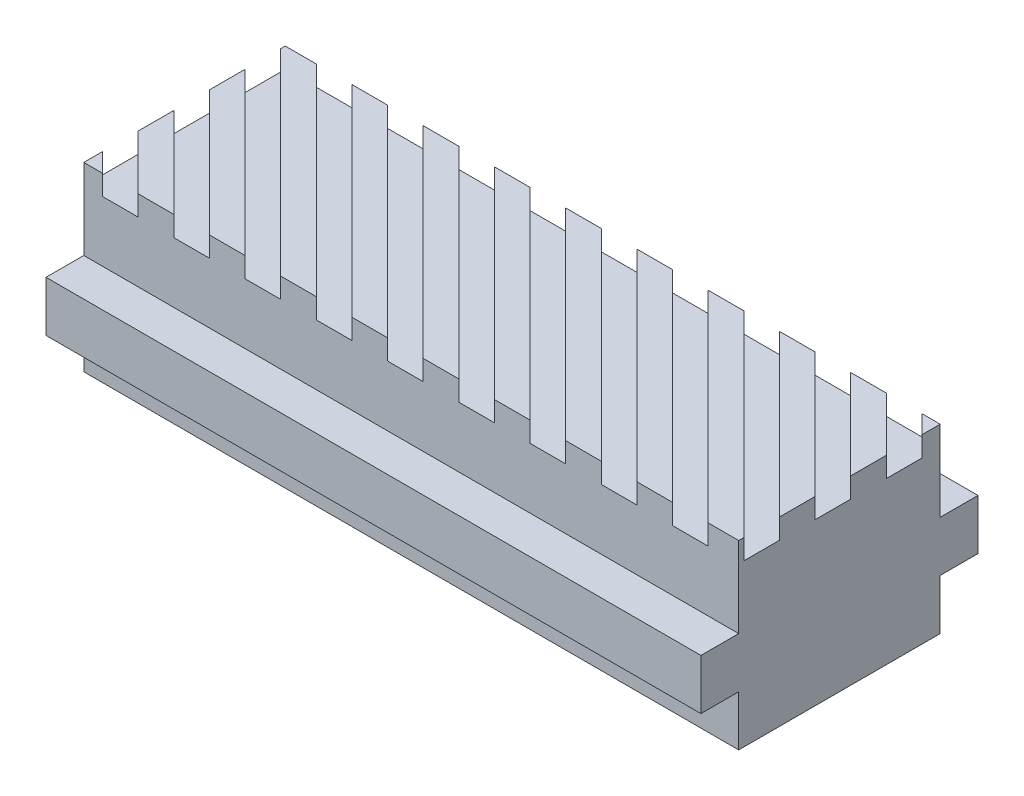
SolidWorks part; units mm, degrees
ref_plane "Front Plane" through (0, 0, 0) normal (0, 0, 1) x (1, 0, 0)
ref_plane "Top Plane" through (0, 0, 0) normal (0, 1, 0) x (1, 0, 0)
ref_plane "Right Plane" through (0, 0, 0) normal (1, 0, 0) x (0, 0, -1)
sketch "Sketch1" plane through (0, 0, 0) normal (0, 1, 0) x (1, 0, 0)
  line L1 (-90, 20) -> (90, 20)
  line L2 (-90, 20) -> (-90, -20)
  line L3 (-90, -20) -> (90, -20)
  line L4 (90, 20) -> (90, -20)
  line L5 (-90, 20) -> (90, -20) construction
  line L6 (-90, -20) -> (90, 20) construction
  point P0 (0, 0)
  dimension "D1" = 40
  dimension "D2" = 180
extrude "Boss-Extrude1" add sketch "Sketch1" along normal blind 6
sketch "Sketch5" plane through (0, 6, 0) normal (0, 1, 0) x (1, 0, 0)
  line L0 (-107.3292, 97.0302) -> (117.2597, -127.5588) construction
  line L1 (-105.5615, 98.7979) -> (119.0275, -125.791)
  line L2 (-109.097, 95.2624) -> (115.492, -129.3266)
  line L3 (90, 20) -> (-90, 20) construction
  line L4 (-8.9821, -1.317) -> (-4.9419, 2.7233) construction
  line L5 (-102.0259, 102.3335) -> (122.563, -122.2555)
  line L6 (-98.4904, 105.869) -> (126.0986, -118.72)
  line L7 (-100.2582, 104.1012) -> (124.3308, -120.4877) construction
  line L8 (-94.9549, 109.4045) -> (129.6341, -115.1844)
  line L9 (-91.4193, 112.9401) -> (133.1696, -111.6489)
  line L10 (-93.1871, 111.1723) -> (131.4019, -113.4167) construction
  line L11 (-87.8838, 116.4756) -> (136.7052, -108.1134)
  line L12 (-84.3483, 120.0111) -> (140.2407, -104.5778)
  line L13 (-86.116, 118.2434) -> (138.4729, -106.3456) construction
  line L14 (-80.8127, 123.5467) -> (143.7762, -101.0423)
  line L15 (-77.2772, 127.0822) -> (147.3118, -97.5068)
  line L16 (-79.045, 125.3144) -> (145.544, -99.2745) construction
  line L17 (-73.7417, 130.6177) -> (150.8473, -93.9712)
  line L18 (-70.2061, 134.1533) -> (154.3828, -90.4357)
  line L19 (-71.9739, 132.3855) -> (152.6151, -92.2035) construction
  line L20 (-66.6706, 137.6888) -> (157.9184, -86.9002)
  line L21 (-63.1351, 141.2243) -> (161.4539, -83.3646)
  line L22 (-64.9028, 139.4566) -> (159.6861, -85.1324) construction
  line L23 (-59.5995, 144.7599) -> (164.9894, -79.8291)
  line L24 (-56.064, 148.2954) -> (168.525, -76.2936)
  line L25 (-57.8318, 146.5276) -> (166.7572, -78.0613) construction
  line L26 (-52.5285, 151.8309) -> (172.0605, -72.758)
  line L27 (-48.9929, 155.3665) -> (175.596, -69.2225)
  line L28 (-50.7607, 153.5987) -> (173.8283, -70.9903) construction
  line L29 (-45.4574, 158.902) -> (179.1316, -65.687)
  line L30 (-41.9219, 162.4375) -> (182.6671, -62.1514)
  line L31 (-43.6896, 160.6698) -> (180.8993, -63.9192) construction
  line L32 (-116.1681, 88.1913) -> (108.4209, -136.3976)
  line L33 (-112.6325, 91.7269) -> (111.9564, -132.8621)
  line L34 (-114.4003, 89.9591) -> (110.1886, -134.6299) construction
  line L35 (-123.2391, 81.1203) -> (101.3498, -143.4687)
  line L36 (-119.7036, 84.6558) -> (104.8853, -139.9332)
  line L37 (-121.4714, 82.888) -> (103.1176, -141.7009) construction
  line L38 (-130.3102, 74.0492) -> (94.2787, -150.5398)
  line L39 (-126.7747, 77.5847) -> (97.8143, -147.0042)
  line L40 (-128.5424, 75.817) -> (96.0465, -148.772) construction
  line L41 (-137.3813, 66.9781) -> (87.2077, -157.6108)
  line L42 (-133.8457, 70.5137) -> (90.7432, -154.0753)
  line L43 (-135.6135, 68.7459) -> (88.9754, -155.8431) construction
  line L44 (-144.4524, 59.9071) -> (80.1366, -164.6819)
  line L45 (-140.9168, 63.4426) -> (83.6721, -161.1464)
  line L46 (-142.6846, 61.6748) -> (81.9044, -162.9141) construction
  line L47 (-151.5234, 52.836) -> (73.0655, -171.753)
  line L48 (-147.9879, 56.3715) -> (76.6011, -168.2174)
  line L49 (-149.7557, 54.6038) -> (74.8333, -169.9852) construction
  line L50 (-158.5945, 45.7649) -> (65.9945, -178.824)
  line L51 (-155.059, 49.3005) -> (69.53, -175.2885)
  line L52 (-156.8267, 47.5327) -> (67.7622, -177.0563) construction
  arc A0 (-105.5615, 98.7979) -> (-109.097, 95.2624) centre (-107.3292, 97.0302) ccw
  arc A1 (115.492, -129.3266) -> (119.0275, -125.791) centre (117.2597, -127.5588) ccw
  arc A2 (-98.4904, 105.869) -> (-102.0259, 102.3335) centre (-100.2582, 104.1012) ccw
  arc A3 (122.563, -122.2555) -> (126.0986, -118.72) centre (124.3308, -120.4877) ccw
  arc A4 (-91.4193, 112.9401) -> (-94.9549, 109.4045) centre (-93.1871, 111.1723) ccw
  arc A5 (129.6341, -115.1844) -> (133.1696, -111.6489) centre (131.4019, -113.4167) ccw
  arc A6 (-84.3483, 120.0111) -> (-87.8838, 116.4756) centre (-86.116, 118.2434) ccw
  arc A7 (136.7052, -108.1134) -> (140.2407, -104.5778) centre (138.4729, -106.3456) ccw
  arc A8 (-77.2772, 127.0822) -> (-80.8127, 123.5467) centre (-79.045, 125.3144) ccw
  arc A9 (143.7762, -101.0423) -> (147.3118, -97.5068) centre (145.544, -99.2745) ccw
  arc A10 (-70.2061, 134.1533) -> (-73.7417, 130.6177) centre (-71.9739, 132.3855) ccw
  arc A11 (150.8473, -93.9712) -> (154.3828, -90.4357) centre (152.6151, -92.2035) ccw
  arc A12 (-63.1351, 141.2243) -> (-66.6706, 137.6888) centre (-64.9028, 139.4566) ccw
  arc A13 (157.9184, -86.9002) -> (161.4539, -83.3646) centre (159.6861, -85.1324) ccw
  arc A14 (-56.064, 148.2954) -> (-59.5995, 144.7599) centre (-57.8318, 146.5276) ccw
  arc A15 (164.9894, -79.8291) -> (168.525, -76.2936) centre (166.7572, -78.0613) ccw
  arc A16 (-48.9929, 155.3665) -> (-52.5285, 151.8309) centre (-50.7607, 153.5987) ccw
  arc A17 (172.0605, -72.758) -> (175.596, -69.2225) centre (173.8283, -70.9903) ccw
  arc A18 (-41.9219, 162.4375) -> (-45.4574, 158.902) centre (-43.6896, 160.6698) ccw
  arc A19 (179.1316, -65.687) -> (182.6671, -62.1514) centre (180.8993, -63.9192) ccw
  arc A20 (-112.6325, 91.7269) -> (-116.1681, 88.1913) centre (-114.4003, 89.9591) ccw
  arc A21 (108.4209, -136.3976) -> (111.9564, -132.8621) centre (110.1886, -134.6299) ccw
  arc A22 (-119.7036, 84.6558) -> (-123.2391, 81.1203) centre (-121.4714, 82.888) ccw
  arc A23 (101.3498, -143.4687) -> (104.8853, -139.9332) centre (103.1176, -141.7009) ccw
  arc A24 (-126.7747, 77.5847) -> (-130.3102, 74.0492) centre (-128.5424, 75.817) ccw
  arc A25 (94.2787, -150.5398) -> (97.8143, -147.0042) centre (96.0465, -148.772) ccw
  arc A26 (-133.8457, 70.5137) -> (-137.3813, 66.9781) centre (-135.6135, 68.7459) ccw
  arc A27 (87.2077, -157.6108) -> (90.7432, -154.0753) centre (88.9754, -155.8431) ccw
  arc A28 (-140.9168, 63.4426) -> (-144.4524, 59.9071) centre (-142.6846, 61.6748) ccw
  arc A29 (80.1366, -164.6819) -> (83.6721, -161.1464) centre (81.9044, -162.9141) ccw
  arc A30 (-147.9879, 56.3715) -> (-151.5234, 52.836) centre (-149.7557, 54.6038) ccw
  arc A31 (73.0655, -171.753) -> (76.6011, -168.2174) centre (74.8333, -169.9852) ccw
  arc A32 (-155.059, 49.3005) -> (-158.5945, 45.7649) centre (-156.8267, 47.5327) ccw
  arc A33 (65.9945, -178.824) -> (69.53, -175.2885) centre (67.7622, -177.0563) ccw
  point P2 (4.9652, -15.2643)
  point P14 (12.0363, -8.1933)
  point P21 (19.1074, -1.1222)
  point P28 (26.1784, 5.9489)
  point P35 (33.2495, 13.02)
  point P42 (40.3206, 20.091)
  point P49 (47.3916, 27.1621)
  point P56 (54.4627, 34.2332)
  point P63 (61.5338, 41.3042)
  point P70 (68.6048, 48.3753)
  point P77 (-2.1058, -22.3354)
  point P84 (-9.1769, -29.4065)
  point P91 (-16.248, -36.4775)
  point P98 (-23.319, -43.5486)
  point P105 (-30.3901, -50.6197)
  point P112 (-37.4612, -57.6907)
  point P119 (-44.5322, -64.7618)
  dimension "D1" = 5
  dimension "D2" = 45
  dimension "D3" = 10
  dimension "D4" = 8
extrude "Cut-Extrude2" cut sketch "Sketch5" against normal blind 4
sketch "Sketch6" plane through (0, 0, 0) normal (0, -1, 0) x (1, 0, 0)
  line L0 (-90, 20) -> (90, 20) construction
  line L1 (-90, -20) -> (90, -20)
  line L3 (-90, 20) -> (90, 20)
  line L4 (90, -20) -> (90, 20)
  line L5 (-90, -20) -> (90, 20) construction
  line L6 (-90, 20) -> (90, -20) construction
  line L7 (-90, 20) -> (-90, -20)
  line L8 (90, 20) -> (90, -20) construction
  point P0 (0, 0)
extrude "Boss-Extrude3" add sketch "Sketch6" along normal blind 30
sketch "Sketch7" plane through (0, -30, 0) normal (0, -1, 0) x (1, 0, 0)
  line L0 (-90, -20) -> (90, -20) construction
  line L1 (-90, 20) -> (-40, 20)
  line L2 (-90, 20) -> (-90, -20)
  line L3 (-90, -20) -> (-40, -20)
  line L4 (-40, 20) -> (-40, -20)
  line L5 (90, -20) -> (90, 20) construction
  dimension "D1" = 130
extrude "Cut-Extrude3" cut sketch "Sketch7" against normal blind 40
sketch "Sketch8" plane through (90, 0, 0) normal (1, 0, 0) x (0, 0, -1)
  line L0 (0, -30) -> (0, 6) construction
  line L1 (20, -30) -> (-20, -30) construction
  line L2 (20, 6) -> (-4.8397, 6) construction
  line L4 (-27.5, -10) -> (27.5, -10)
  line L5 (-27.5, -10) -> (-27.5, -20)
  line L6 (-27.5, -20) -> (27.5, -20)
  line L7 (27.5, -10) -> (27.5, -20)
  line L8 (-27.5, -10) -> (27.5, -20) construction
  line L9 (-27.5, -20) -> (27.5, -10) construction
  point P7 (0, -15)
  dimension "D1" = 10
  dimension "D2" = 55
  dimension "D3" = 10
extrude "Boss-Extrude4" add sketch "Sketch8" against normal through all
sketch "Sketch9" plane through (0, -30, 0) normal (0, -1, 0) x (1, 0, 0)
  line L0 (-40, 0) -> (90, 0) construction
  line L1 (-40, -20) -> (-40, 20) construction
  line L2 (90, -20) -> (90, 20) construction
  circle A0 centre (60, 0) radius 7.5
  circle A1 centre (-10, 0) radius 7.5
  dimension "D1" = 15
  dimension "D2" = 15
  dimension "D4" = 30
  dimension "D3" = 30
extrude "Cut-Extrude4" cut sketch "Sketch9" against normal blind 25
